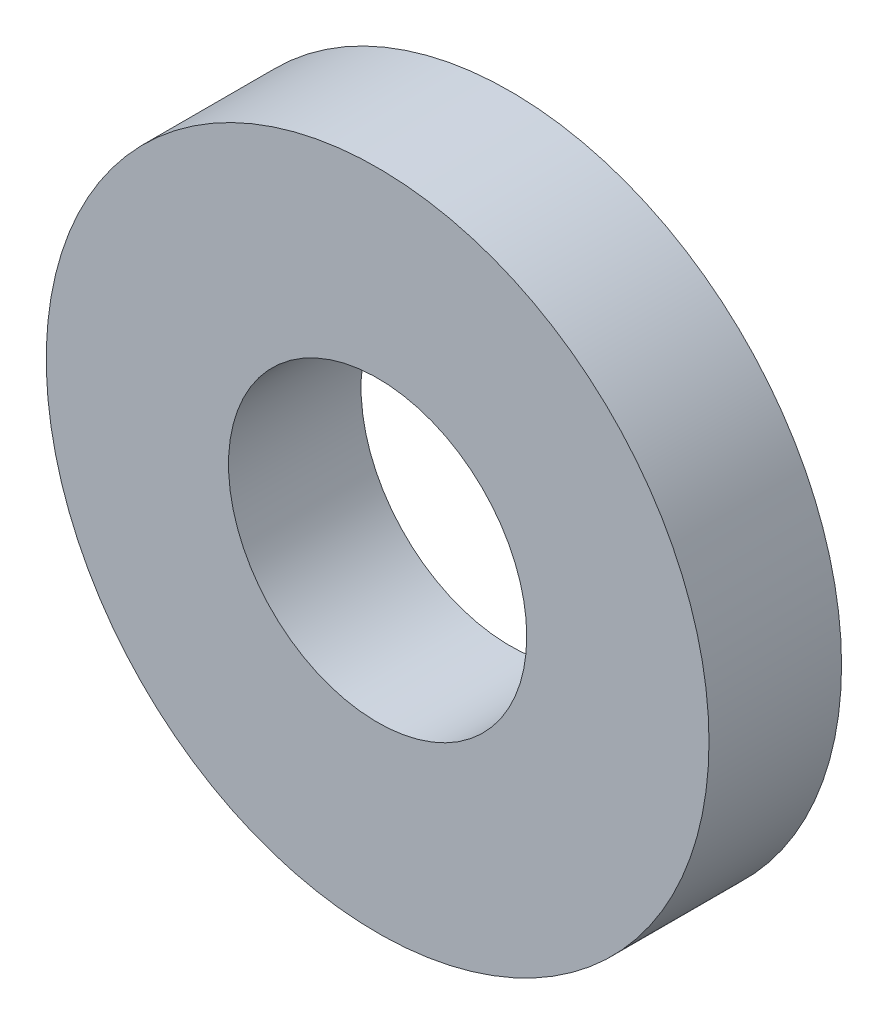
SolidWorks part; units mm, degrees
material "聚亚安酯(11671)"
ref_plane "前视基准面" through (0, 0, 0) normal (0, 0, 1) x (1, 0, 0)
ref_plane "上视基准面" through (0, 0, 0) normal (0, 1, 0) x (1, 0, 0)
ref_plane "右视基准面" through (0, 0, 0) normal (1, 0, 0) x (0, 0, -1)
sketch "草图1" plane through (0, 0, 0) normal (0, 0, 1) x (1, 0, 0)
  circle A0 centre (0, 0) radius 4.5
  circle A1 centre (0, 0) radius 10
  dimension "D1" = 9
  dimension "D2" = 20
extrude "凸台-拉伸1" add sketch "草图1" along normal blind 4
